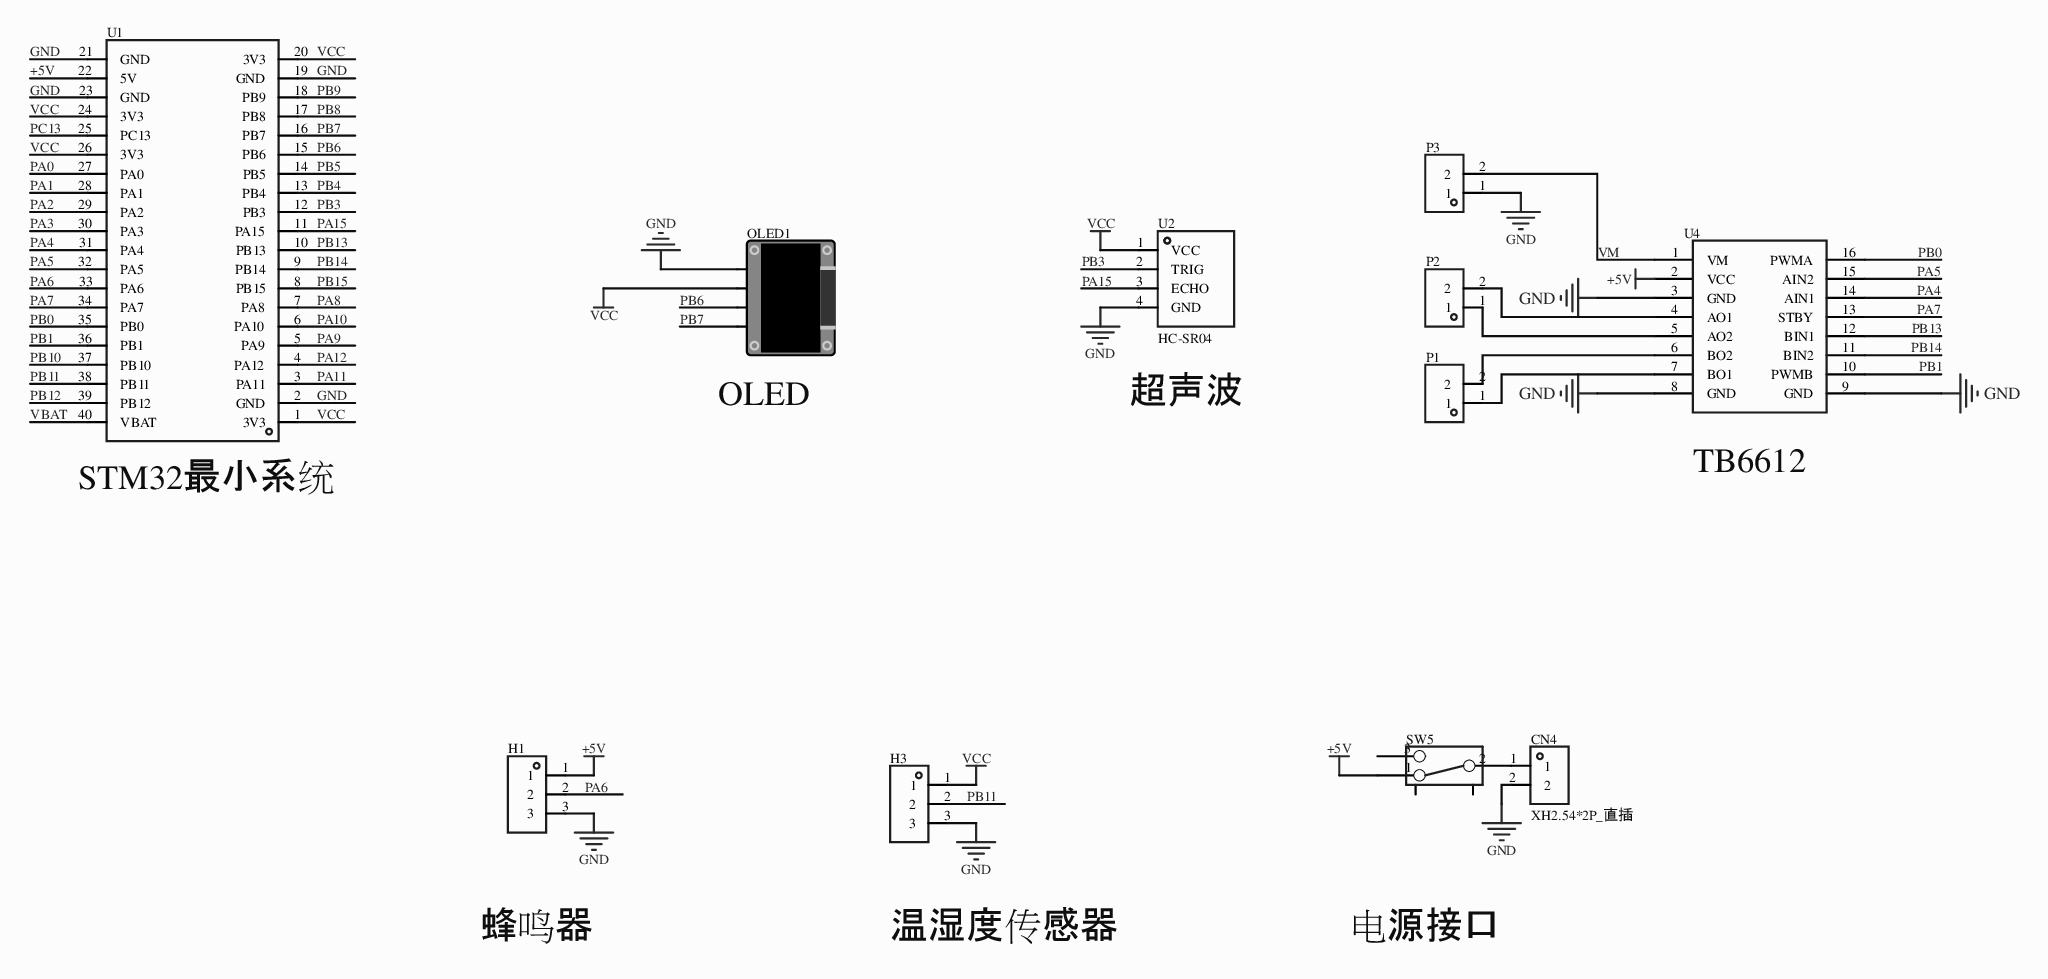
[diagram p0: MISC52080-3.schdoc]
# Altium project MISC52080-2.PrjPcb
1 sheet, 11 parts. Net scope: global (net labels, ports and power ports of the same name join across sheets).
Board file: MISC52080.pcbdoc

## Sheet MISC52080-3.schdoc
size 297 x 209 mm; Version: V1.0; @Project Name: MISC52080; @Page Count: 1; @Update Date: 2026-04-28; @Create Date: 2026-04-28; @Schematic Name: MISC52080; @Page No: 1; @Create Time: 23:22:16; @Update Time: 17:32:40; @Board Name: MISC52080

### Parts
CN4  XH2.54*2P_直插  [CONN-TH_2P-P2.50-XH2.54-2P]
H1  (no value)  [HDR-TH_3P-P2.54-V-F]
H3  (no value)  [HDR-TH_3P-P2.54-V-F]
OLED1  (no value)  [0.96OLED_4P]
P1  KF301-2P接线端子  [CONN-TH_XY301V-A-5.0-2P]  (value not drawn)
P2  KF301-2P接线端子  [CONN-TH_XY301V-A-5.0-2P]  (value not drawn)
P3  KF301-2P接线端子  [CONN-TH_XY301V-A-5.0-2P]  (value not drawn)
SW5  (no value)  [拨动开关]
U1  STM32F103C8T6-Card  [CONN-TH_L53.3-W22.9_STM32F103C8T6-CARD]  (value not drawn)
U2  HC-SR04  [TH_HC-SR04V]
U4  (no value)  [tb6612]

### Nets
+5V: H1.1 SW5.1 U1.22(5V) U4.2(VCC)
GND: CN4.2 H1.3 H3.3 OLED1.1(GND) P3.1 U1.2(GND) U1.19(GND) U1.21(GND) U1.23(GND) U2.4(GND) U4.3(GND) U4.8(GND) U4.9(GND)
VCC: H3.1 OLED1.2(VCC) U1.1(3V3) U1.20(3V3) U1.24(3V3) U1.26(3V3) U2.1(VCC)
PA0: U1.27(PA0)
PA1: U1.28(PA1)
PA2: U1.29(PA2)
PA3: U1.30(PA3)
PA4: U1.31(PA4) U4.14(AIN1)
PA5: U1.32(PA5) U4.15(AIN2)
PA6: H1.2 U1.33(PA6)
PA7: U1.34(PA7) U4.13(STBY)
PA8: U1.7(PA8)
PA9: U1.5(PA9)
PA10: U1.6(PA10)
PA11: U1.3(PA11)
PA12: U1.4(PA12)
PA15: U1.11(PA15) U2.3(ECHO)
PB0: U1.35(PB0) U4.16(PWMA)
PB1: U1.36(PB1) U4.10(PWMB)
PB3: U1.12(PB3) U2.2(TRIG)
PB4: U1.13(PB4)
PB5: U1.14(PB5)
PB6: OLED1.3(SCL) U1.15(PB6)
PB7: OLED1.4(SDA) U1.16(PB7)
PB8: U1.17(PB8)
PB9: U1.18(PB9)
PB10: U1.37(PB10)
PB11: H3.2 U1.38(PB11)
PB12: U1.39(PB12)
PB13: U1.10(PB13) U4.12(BIN1)
PB14: U1.9(PB14) U4.11(BIN2)
PB15: U1.8(PB15)
PC13: U1.25(PC13)
VBAT: U1.40(VBAT)
VM: P3.2 U4.1(VM)
NetCN4_1: CN4.1 SW5.2
NetP1_1: P1.1 U4.7(BO1)
NetP1_2: P1.2 U4.6(BO2)
NetP2_1: P2.1 U4.5(AO2)
NetP2_2: P2.2 U4.4(AO1)

Not connected (* = marked no-connect by the designer): SW5 3 4 5

### Notes on the sheet
- (near OLED1) OLED
- (near U2) 超声波
- (near U4) TB6612
- (near U1) STM32最小系统
- 蜂鸣器
- 温湿度传感器
- 电源接口

### Library data of the parts
CN4 = XH2.54*2P_直插: 3D Model: 325c595e30db4df8abe76612dd40b0fa0819f05c4eef4c71ace90d822a990e87; 3D Model Transform: 295.275,228.346,0,180,0,0,-0.002,-20.079,-137.795; AddInBom: yes; Symbol: XH2.54*2P_直插; Device: XH2.54*2P_直插; LCSC Part Name: XH2.54*2P_直插; Supplier Part: C9900008615; Manufacturer Part: XH2.54*2P_直插; Supplier Footprint: XH2.54_2P; JLCPCB Part Class: Extended Part; Supplier: LCSC; FootprintName: CONN-TH_2P-P2.50-XH2.54-2P; ConvertToPcb: yes; ModelName: CONN-TH_2P-P2.50-XH2.54-2P
H1 H3 = HDR-F_2.54_1x3P: Symbol: PM254V-11-03-H85; 3D Model: f3b3cc5aae9641bf9e56fc160cef875b; 3D Model Transform: 299.9994,100,0,0,0,0,0,0,-118.11; ConvertToPcb: yes; ModelName: HDR2.54-F-LI-1X3P; Device: HDR-F_2.54_1x3P; Supplier Part: C541850; Supplier Footprint: 插件; FootprintName: HDR-TH_3P-P2.54-V-F; AddInBom: yes
OLED1 = 0.96OLED模块_4P: 3D Model: 79c000fdb68d45a296c2e9bedf4f9055; 3D Model Transform: 1393.69792,1318.895,0,0,0,0,0,-560.079,-137.795; ConvertToPcb: yes; Symbol: 0.96OLED模块_4P; Device: 0.96OLED模块_4P; Supplier Footprint: 插件; AddInBom: yes; FootprintName: 0.96OLED_4P; ModelName: 0.96OLED_4P
P1-P3 = KF301-2P接线端子: 3D Model: ef7ead88b0f2448d904975b26718870f; 3D Model Transform: 417.322,299.212,0,0,0,0,11.811,-7.835,-157.48; AddInBom: yes; Symbol: KF301-2P接线端子; Device: KF301-2P接线端子; LCSC Part Name: KF301-2P接线端子; Supplier Part: C9900016950; Manufacturer Part: KF301-2P接线端子; Supplier Footprint: CK301-2P; Supplier: LCSC; ConvertToPcb: yes; FootprintName: CONN-TH_XY301V-A-5.0-2P; ModelName: CONN-TH_XY301V-A-5.0-2P
SW5 = 拨动开关_正: 3D Model: 4321fe59a4074cbfb4989553f297c68f0819f05c4eef4c71ace90d822a990e87; 3D Model Transform: 370.09,208.7,472.35,0,0,0,0,0,-110; ConvertToPcb: yes; ModelName: SW-TH_SS-12D02-VG4; Symbol: 拨动开关; Device: 拨动开关_正; Supplier Footprint: 插件; FootprintName: 拨动开关; AddInBom: yes
U1 = STM32F103C8T6-Card: AddInBom: yes; Device: STM32F103C8T6-Card; Symbol: STM32F103C8T6-CARD; FootprintName: CONN-TH_L53.3-W22.9_STM32F103C8T6-CARD; LCSC Part Name: STM32F103C8T6-Card; SupplierPart: C9900077949; ManufacturerPart: STM32F103C8T6-Card; Supplier Footprint: 插件; Supplier: LCSC; ConvertToPcb: yes
U2 = HC-SR04: Manufacturer: Universal Microelectronics; AddInBom: yes; Symbol: HC-SR04; Device: HC-SR04; LCSC Part Name: HC-SR04; SupplierPart: C19857336; ManufacturerPart: HC-SR04; Supplier Footprint: -; JLCPCB Part Class: 扩展库; Datasheet: https://atta.szlcsc.com/upload/public/pdf/source/20240122/47B8E374E428935B7962A2189EF91AAC.pdf; Supplier: LCSC; ConvertToPcb: yes; FootprintName: TH_HC-SR04V
U4 = tb6612: AddInBom: yes; Symbol: tb6612; Device: tb6612; JLCPCB Part Class: 扩展库; ConvertToPcb: yes; FootprintName: tb6612